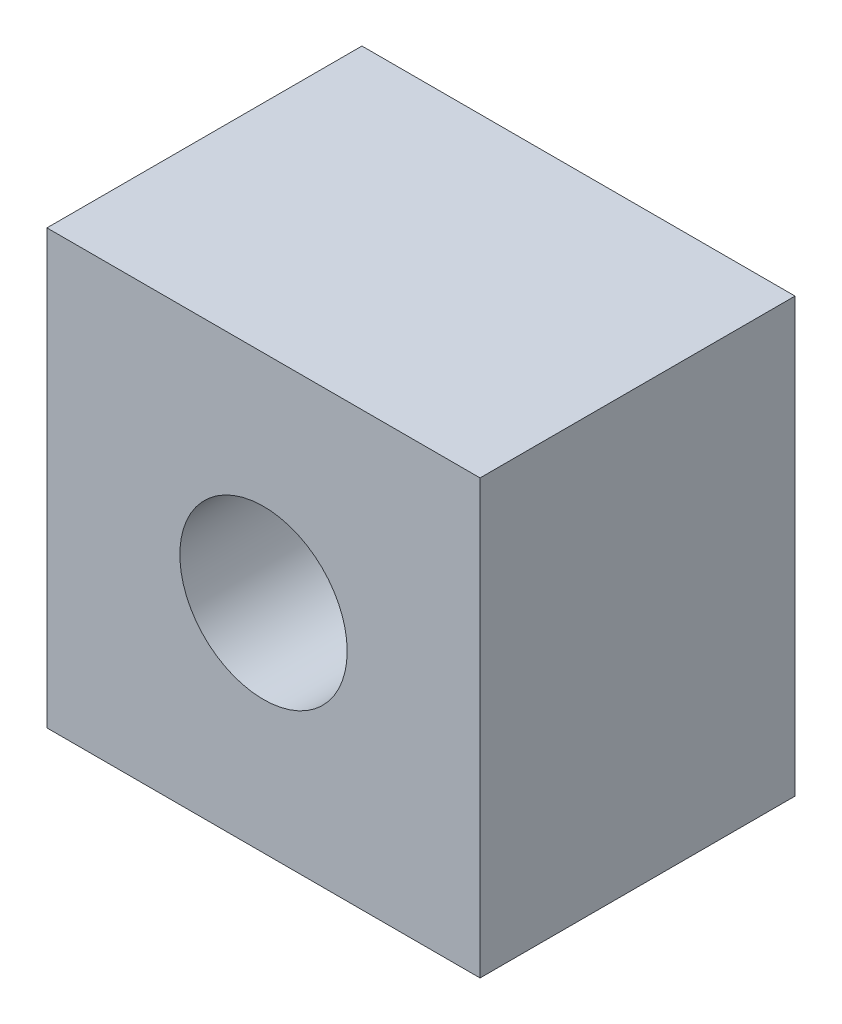
SolidWorks part; units mm, degrees
material "SS400B"
ref_plane "Front Plane" through (0, 0, 0) normal (0, 0, 1) x (1, 0, 0)
ref_plane "Top Plane" through (0, 0, 0) normal (0, 1, 0) x (1, 0, 0)
ref_plane "Right Plane" through (0, 0, 0) normal (1, 0, 0) x (0, 0, -1)
sketch "Sketch1" plane through (0, 0, 0) normal (0, 0, 1) x (1, 0, 0)
  line L1 (-11, 11) -> (11, 11)
  line L2 (-11, 11) -> (-11, -11)
  line L3 (-11, -11) -> (11, -11)
  line L4 (11, 11) -> (11, -11)
  line L5 (-11, 11) -> (11, -11) construction
  line L6 (-11, -11) -> (11, 11) construction
  point P0 (0, 0)
  dimension "D1" = 22
  dimension "D2" = 22
extrude "Boss-Extrude1" add sketch "Sketch1" along normal blind 16
hole_wizard "M10 Tapped Hole1" positions "Sketch2" profile "Sketch3" tap size "M10" standard "GB"
sketch "Sketch2" plane through (0, 0, 16) normal (0, 0, 1) x (1, 0, 0)
  point P0 (0, 0)
sketch "Sketch3" plane through (0, 0, 16) normal (1, 0, 0) x (0, -1, 0)
  line L0 (0, 0) -> (0, 30.0537)
  line L1 (0, 30.0537) -> (4.25, 27.5)
  line L2 (4.25, 27.5) -> (4.25, 0)
  line L5 (4.25, 0) -> (0, 0)
  line L10 (0, 30.0537) -> (-4.25, 27.5) construction
  line L11 (0, -6.35) -> (0, 107.95) construction
  dimension "螺纹孔钻头直径" = 8.5
  dimension "螺纹孔钻头深度" = 27.5
  dimension "导头角度" = 118
cosmetic thread "Cosmetic Thread 1" parameters "D1"=20, "D2"=10
